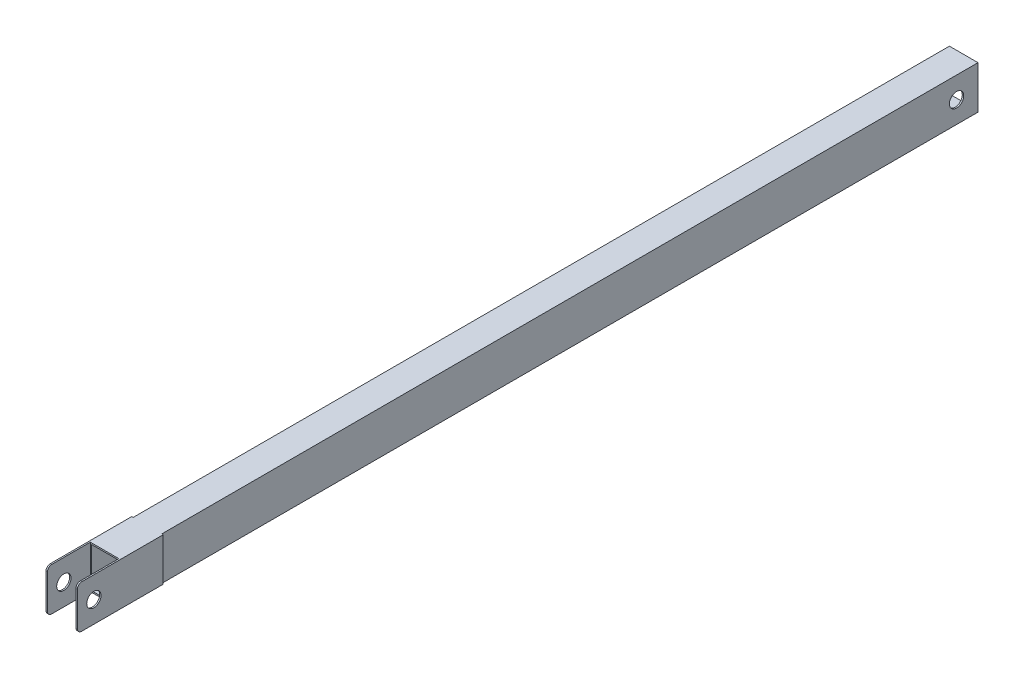
SolidWorks part; units mm, degrees
ref_plane "Front Plane" through (0, 0, 0) normal (0, 0, 1) x (1, 0, 0)
ref_plane "Top Plane" through (0, 0, 0) normal (0, 1, 0) x (1, 0, 0)
ref_plane "Right Plane" through (0, 0, 0) normal (1, 0, 0) x (0, 0, -1)
sketch "Sketch1" plane through (0, 0, 0) normal (0, 0, 1) x (1, 0, 0)
  line L1 (0, 0) -> (20, 0)
  line L2 (0, 0) -> (0, -30)
  line L3 (0, -30) -> (20, -30)
  line L4 (20, 0) -> (20, -30)
  line L8 (1, -1) -> (19, -1)
  line L9 (19, -1) -> (19, -29)
  line L10 (1, -29) -> (19, -29)
  line L11 (1, -1) -> (1, -29)
  dimension "D1" = 20
  dimension "D2" = 30
  dimension "D3" = 1
extrude "Boss-Extrude1" add sketch "Sketch1" along normal blind 601
sketch "Sketch3" plane through (0, 0, 0) normal (-1, 0, 0) x (0, 0, 1)
  line L0 (571, -30) -> (601, -30)
  line L2 (631, -27) -> (631, -3)
  line L3 (628, 0) -> (601, 0)
  line L4 (601, 0) -> (571, 0)
  line L5 (601, 0) -> (0, 0) construction
  line L6 (601, -30) -> (0, -30) construction
  line L7 (601, -30) -> (628, -30)
  line L8 (571, -30) -> (571, 0)
  arc A0 (631, -27) -> (628, -30) centre (628, -27) cw
  arc A1 (631, -3) -> (628, 0) centre (628, -3) ccw
  point P14 (631, -30)
  dimension "D3" = 3
  dimension "D4" = 3
  dimension "D1" = 30
  dimension "D2" = 30
extrude "Boss-Extrude2" add sketch "Sketch3" along normal blind 1
ref_plane "Plane4" through (10, 0, 0) normal (1, 0, 0) x (0, 0, -1)
mirror "Mirror2" about plane through (10, 0, 0) normal (1, 0, 0) of "Boss-Extrude2"
sketch "Sketch4" plane through (21, 0, 0) normal (1, 0, 0) x (0, 0, -1)
  line L0 (-631, -15) -> (-571, -15) construction
  line L1 (-631, -27) -> (-631, -3) construction
  line L2 (-571, 0) -> (-571, -30) construction
  line L3 (-599.5, 0) -> (-599.5, -30) construction
  line L4 (-628, 0) -> (-571, 0) construction
  line L5 (-571, -30) -> (-628, -30) construction
  circle A0 centre (-619.5, -15) radius 5
  dimension "D2" = 10
  dimension "D1" = 20
extrude "Cut-Extrude1" cut sketch "Sketch4" against normal through all
sketch "Sketch5" plane through (0, 0, 0) normal (-1, 0, 0) x (0, 0, 1)
  line L0 (0, -15) -> (571, -15) construction
  line L1 (0, 0) -> (0, -30) construction
  line L2 (571, 0) -> (571, -30) construction
  circle A0 centre (15, -15) radius 5
  dimension "D1" = 10
  dimension "D2" = 15
extrude "Cut-Extrude2" cut sketch "Sketch5" against normal through all
